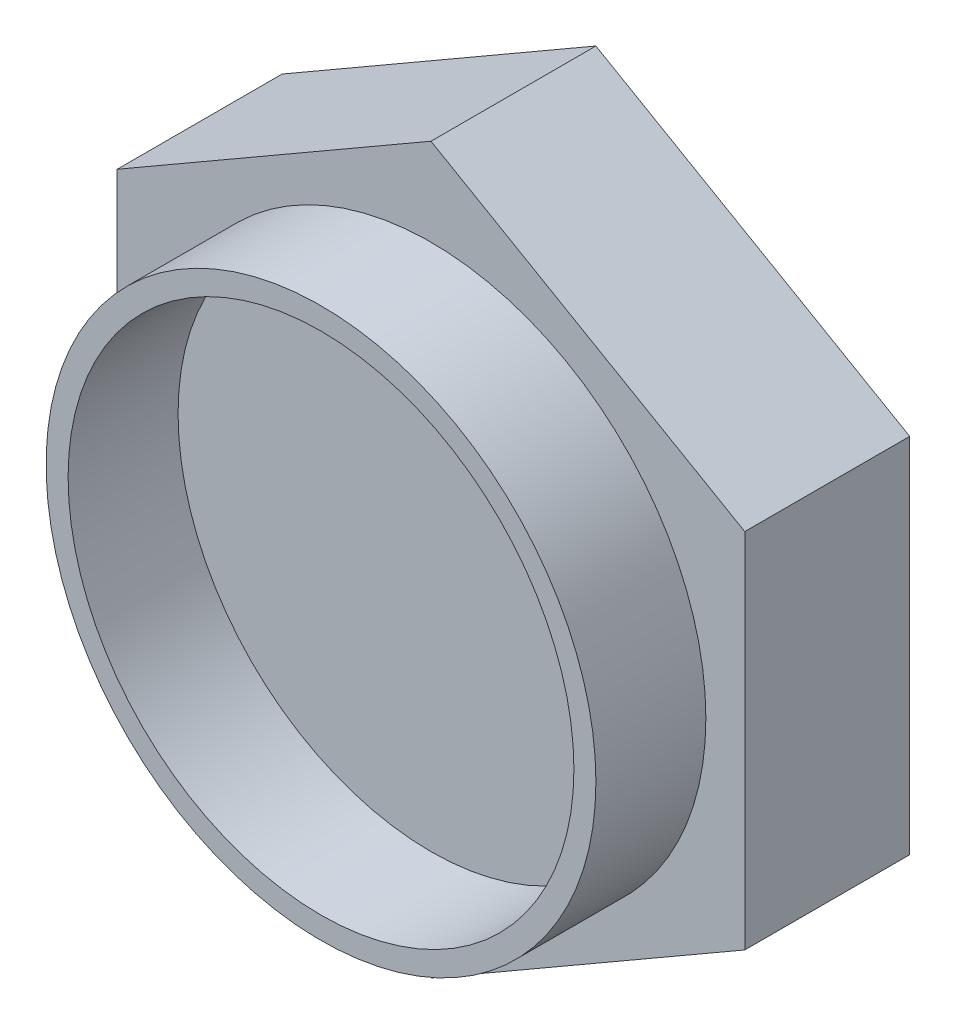
SolidWorks part; units mm, degrees
ref_plane "Front Plane" through (0, 0, 0) normal (0, 0, 1) x (1, 0, 0)
ref_plane "Top Plane" through (0, 0, 0) normal (0, 1, 0) x (1, 0, 0)
ref_plane "Right Plane" through (0, 0, 0) normal (1, 0, 0) x (0, 0, -1)
sketch "Sketch1" plane through (0, 0, 0) normal (0, 0, 1) x (1, 0, 0)
  circle A0 centre (0, 0) radius 25
  circle A1 centre (0, 0) radius 23
  dimension "D1" = 50
  dimension "D2" = 2
extrude "Boss-Extrude1" add sketch "Sketch1" along normal blind 10
sketch "Sketch2" plane through (0, 0, 0) normal (0, 0, -1) x (-1, 0, 0)
  line L1 (0, 32.951) -> (-28.5364, 16.4755)
  line L2 (-28.5364, 16.4755) -> (-28.5364, -16.4755)
  line L3 (-28.5364, -16.4755) -> (0, -32.951)
  line L4 (0, -32.951) -> (28.5364, -16.4755)
  line L5 (28.5364, -16.4755) -> (28.5364, 16.4755)
  line L6 (28.5364, 16.4755) -> (0, 32.951)
  circle A0 centre (0, 0) radius 28.5364 construction
extrude "Boss-Extrude2" add sketch "Sketch2" along normal blind 15
